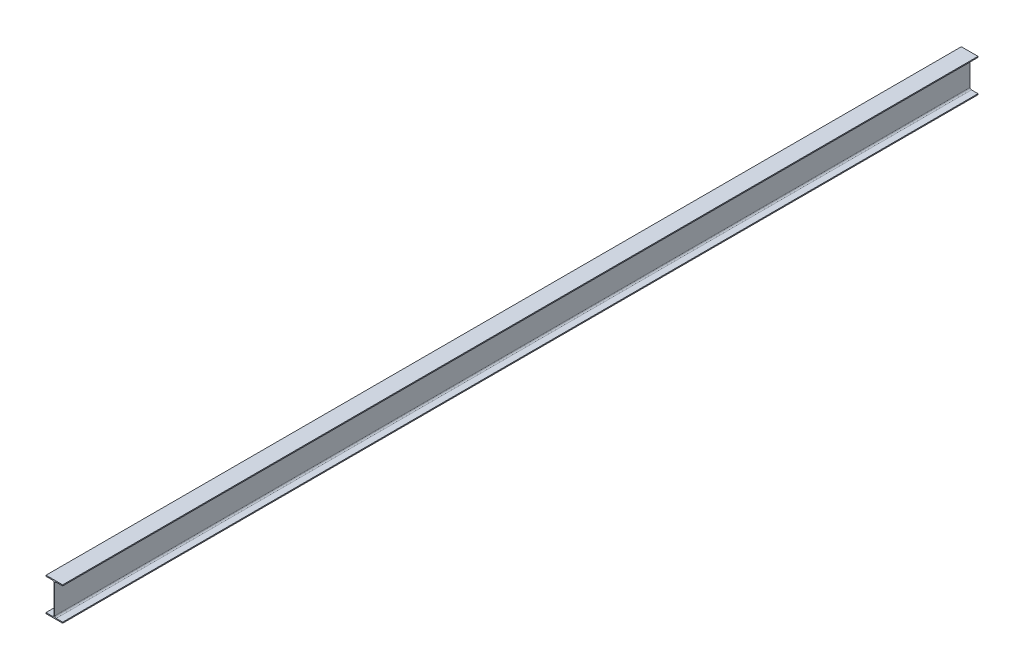
from build123d import *

# Parameters (mm, degrees)
BOSS_EXTRUDE1_DEPTH = 8240


with BuildPart() as part:
    # Sketch1 → Boss-Extrude1 (new body)
    with BuildSketch(Plane.XY):
        with BuildLine():
            Line((75, 0), (-75, 0))
            Line((-75, 0), (-75, 9))
            Line((-75, 9), (-16.25, 9))
            ThreePointArc((-16.25, 9), (-7.057611845, 12.807611845), (-3.25, 22))
            Line((-3.25, 22), (-3.25, 278))
            ThreePointArc((-3.25, 278), (-7.057611845, 287.192388155), (-16.25, 291))
            Line((-16.25, 291), (-75, 291))
            Line((-75, 291), (-75, 300))
            Line((-75, 300), (75, 300))
            Line((75, 300), (75, 291))
            Line((75, 291), (16.25, 291))
            ThreePointArc((16.25, 291), (7.057611845, 287.192388155), (3.25, 278))
            Line((3.25, 278), (3.25, 22))
            ThreePointArc((3.25, 22), (7.057611845, 12.807611845), (16.25, 9))
            Line((16.25, 9), (75, 9))
            Line((75, 9), (75, 0))
        make_face()
    extrude(amount=BOSS_EXTRUDE1_DEPTH)


solid = part.part
